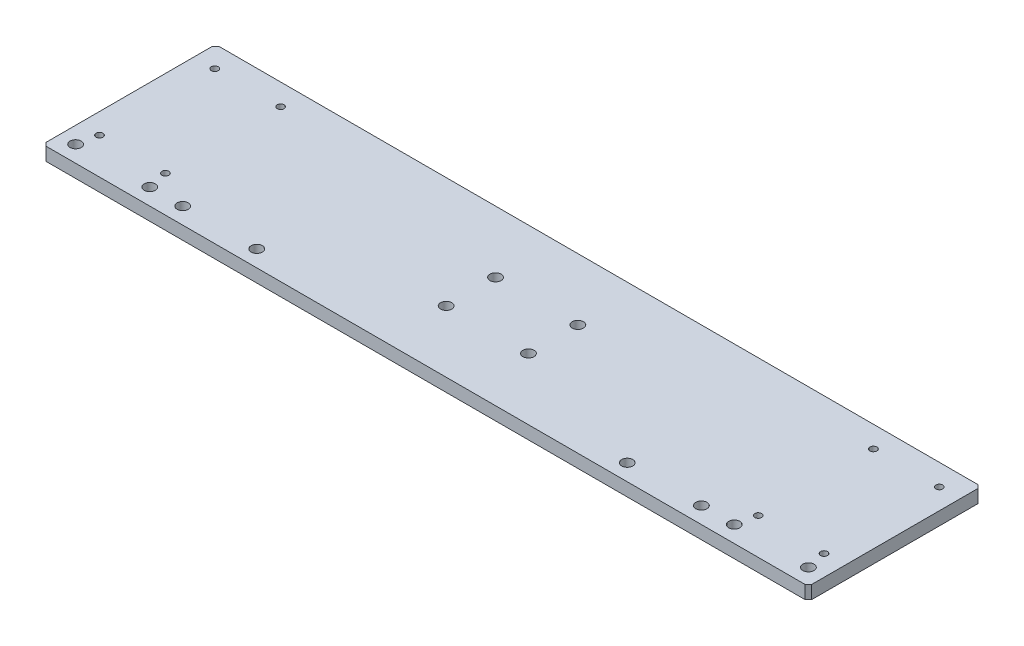
SolidWorks part; units mm, degrees
material "A6061"
ref_plane "前基準面" through (0, 0, 0) normal (0, 0, 1) x (1, 0, 0)
ref_plane "上基準面" through (0, 0, 0) normal (0, 1, 0) x (1, 0, 0)
ref_plane "右基準面" through (0, 0, 0) normal (1, 0, 0) x (0, 0, -1)
sketch "草图1" plane through (0, 0, 0) normal (0, 1, 0) x (1, 0, 0)
  line L1 (-232.5, -52.5) -> (232.5, -52.5)
  line L2 (-232.5, -52.5) -> (-232.5, 52.5)
  line L3 (-232.5, 52.5) -> (232.5, 52.5)
  line L4 (232.5, -52.5) -> (232.5, 52.5)
  line L5 (-232.5, -52.5) -> (232.5, 52.5) construction
  line L6 (-232.5, 52.5) -> (232.5, -52.5) construction
  point P0 (0, 0)
  dimension "D1" = 465
  dimension "D2" = 105
extrude "凸台-拉伸1" add sketch "草图1" along normal mid plane 8
chamfer "倒角1" distance 2 angle 45 4 edges at (232.5, 0, -52.5) (232.5, 0, 52.5) (-232.5, 0, -52.5) (-232.5, 0, 52.5)
hole_wizard "M5 螺纹孔1" positions "草图2" profile "草图3" tap size "M5" standard "GB" end condition through all
sketch "草图2" plane through (0, 4, 0) normal (0, 1, 0) x (1, 0, 0)
  line L0 (0, 107.0949) -> (0, 4.5) construction
  line L1 (0, 4.5) -> (-256.7344, 4.5) construction
  line L3 (230.5, 52.5) -> (-230.5, 52.5) construction
  point P0 (-220, 39.5)
  point P2 (-180, 39.5)
  point P10 (-180, -30.5)
  point P11 (-220, -30.5)
  point P12 (220, -30.5)
  point P13 (180, -30.5)
  point P14 (180, 39.5)
  point P15 (220, 39.5)
  dimension "D1" = 40
  dimension "D2" = 70
  dimension "D3" = 400
  dimension "D4" = 13
sketch "草图3" plane through (-220, 4, -39.5) normal (1, 0, 0) x (0, 0, 1)
  line L0 (0, 0) -> (0, 8)
  line L1 (0, 8) -> (2.1, 8)
  line L2 (2.1, 8) -> (2.1, 0)
  line L5 (2.1, 0) -> (0, 0)
  line L11 (0, -6.35) -> (0, 107.95) construction
  dimension "通孔螺纹孔钻头直径" = 4.2
  dimension "通孔螺纹孔钻头深度" = 8
cosmetic thread "孔螺蚊线1"
cosmetic thread "孔螺蚊线2"
cosmetic thread "孔螺蚊线3"
cosmetic thread "孔螺蚊线4"
cosmetic thread "孔螺蚊线5"
cosmetic thread "孔螺蚊线6"
cosmetic thread "孔螺蚊线7"
cosmetic thread "孔螺蚊线8"
hole_wizard "Ø6.8 (6.8) 直径孔1" positions "草图4" profile "草图5" hole size "Ø6.8" standard "GB" end condition through all
sketch "草图4" plane through (0, 4, 0) normal (0, 1, 0) x (1, 0, 0)
  line L0 (0, 81.503) -> (0, 0) construction
  line L1 (230.5, 52.5) -> (-230.5, 52.5) construction
  point P0 (25, -15)
  point P2 (25, 15)
  point P11 (-25, 15)
  point P12 (-25, -15)
  dimension "D1" = 50
  dimension "D2" = 30
  dimension "D3" = 37.5
sketch "草图5" plane through (25, 4, 15) normal (1, 0, 0) x (0, 0, 1)
  line L0 (0, 0) -> (0, 8)
  line L1 (0, 8) -> (3.4, 8)
  line L2 (3.4, 8) -> (3.4, 0)
  line L5 (3.4, 0) -> (0, 0)
  line L11 (0, -6.35) -> (0, 107.95) construction
  dimension "通孔孔直径" = 6.8
  dimension "通孔孔深度" = 8
hole_wizard "M8 螺纹孔1" positions "草图6" profile "草图7" tap size "M8" standard "GB" end condition through all
sketch "草图6" plane through (0, 4, 0) normal (0, 1, 0) x (1, 0, 0)
  line L0 (0, 0) -> (0, -71.3709) construction
  line L2 (-230.5, -52.5) -> (230.5, -52.5) construction
  line L3 (180, -30.5) -> (220, -30.5) construction
  line L5 (200, -30.5) -> (200, -59.1828) construction
  point P0 (222.5, -42.5)
  point P2 (177.5, -42.5)
  point P8 (-177.5, -42.5)
  point P9 (-222.5, -42.5)
  point P19 (157.5, -42.5)
  point P21 (112.5, -42.5)
  point P24 (-112.5, -42.5)
  point P25 (-157.5, -42.5)
sketch "草图7" plane through (222.5, 4, 42.5) normal (1, 0, 0) x (0, 0, 1)
  line L0 (0, 0) -> (0, 8)
  line L1 (0, 8) -> (3.4, 8)
  line L2 (3.4, 8) -> (3.4, 0)
  line L5 (3.4, 0) -> (0, 0)
  line L11 (0, -6.35) -> (0, 107.95) construction
  dimension "通孔螺纹孔钻头直径" = 6.8
  dimension "通孔螺纹孔钻头深度" = 8
cosmetic thread "孔螺蚊线9"
cosmetic thread "孔螺蚊线10"
cosmetic thread "孔螺蚊线11"
cosmetic thread "孔螺蚊线12"
cosmetic thread "孔螺蚊线13"
cosmetic thread "孔螺蚊线14"
cosmetic thread "孔螺蚊线15"
cosmetic thread "孔螺蚊线16"
equation "\"D4@草图6\"=\"D1@草图6\""
